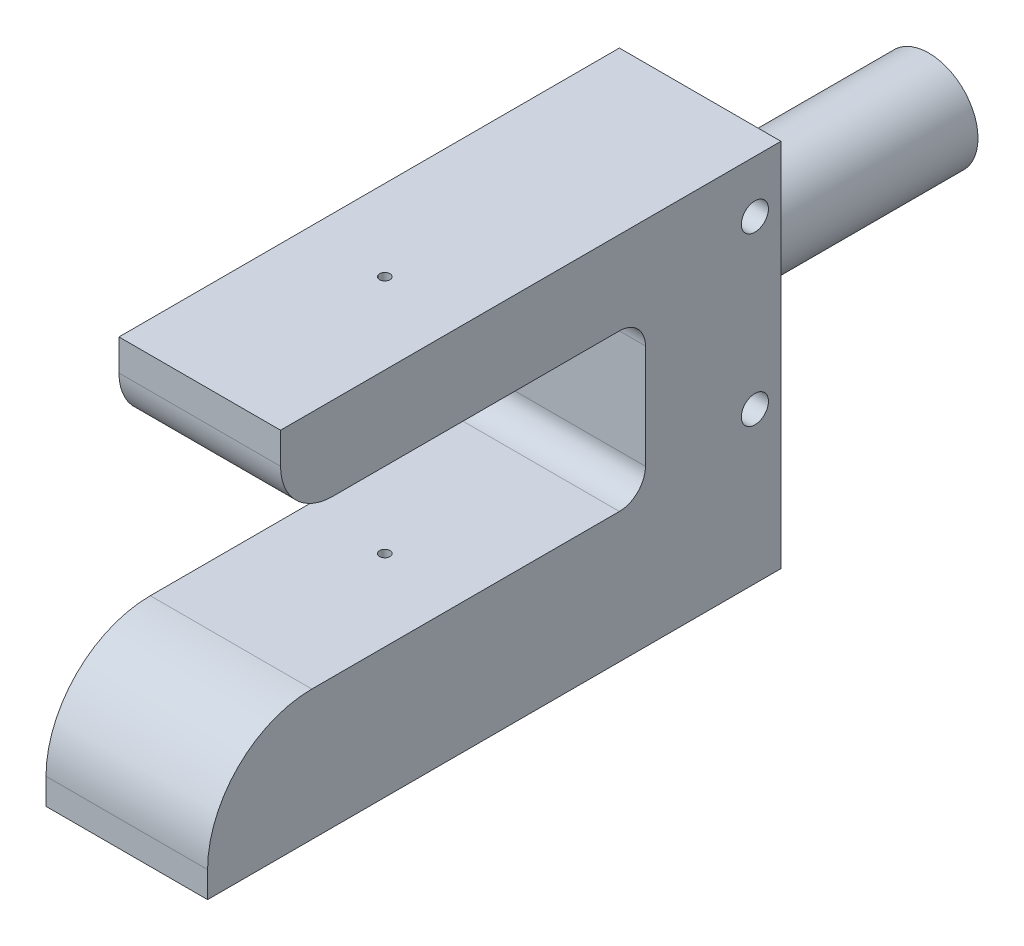
SolidWorks part; units mm, degrees
ref_plane "前视基准面" through (0, 0, 0) normal (0, 0, 1) x (1, 0, 0)
ref_plane "上视基准面" through (0, 0, 0) normal (0, 1, 0) x (1, 0, 0)
ref_plane "右视基准面" through (0, 0, 0) normal (1, 0, 0) x (0, 0, -1)
sketch "草图1" plane through (0, 0, 0) normal (1, 0, 0) x (0, 0, -1)
  line L0 (-55.3793, 24.9576) -> (14.6207, 24.9576)
  line L1 (-55.3793, 40.9576) -> (40.6207, 40.9576)
  line L2 (-55.3793, 40.9576) -> (-55.3793, 24.9576)
  line L3 (-69.3793, -30.0424) -> (40.6207, -30.0424)
  line L4 (40.6207, 40.9576) -> (40.6207, -30.0424)
  line L5 (-55.3793, 40.9576) -> (40.6207, -30.0424) construction
  line L6 (-38.0184, -38.3337) -> (40.6207, 40.9576) construction
  line L7 (14.6207, 24.9576) -> (14.6207, -5.0424)
  line L8 (14.6207, -5.0424) -> (-69.3793, -5.0424)
  line L9 (-69.3793, -5.0424) -> (-69.3793, -30.0424)
  point P0 (0, 0)
  dimension "D1" = 110
  dimension "D2" = 96
  dimension "D3" = 71
  dimension "D4" = 30
  dimension "D5" = 16
  dimension "D6" = 70
extrude "凸台-拉伸1" add sketch "草图1" along normal blind 31
sketch "草图2" plane through (0, 40.9576, 0) normal (0, 1, 0) x (1, 0, 0)
  line L0 (15.5, -69.3793) -> (15.5, 5.5421) construction
  line L1 (31, -69.3793) -> (0, -69.3793) construction
  line L2 (31, -55.3793) -> (0, -55.3793) construction
  circle A0 centre (15.5, -19.8793) radius 1
  dimension "D2" = 2
  dimension "D1" = 35.5
extrude "切除-拉伸1" cut sketch "草图2" against normal through all
fillet "圆角1" radius 10 1 edges at (15.5, 24.9576, 55.3793)
fillet "圆角2" radius 20 1 edges at (15.5, -5.0424, 69.3793)
fillet "圆角3" radius 5 2 edges at (15.5, -5.0424, -14.6207) (15.5, 24.9576, -14.6207)
hole_wizard "Ø5.2 (5.2) 直径孔1" positions "草图3" profile "草图4" hole size "Ø5.2" standard "GB"
sketch "草图3" plane through (31, 0, 0) normal (1, 0, 0) x (0, 0, -1)
  line L0 (40.6207, -30.0424) -> (40.6207, 40.9576) construction
  line L1 (40.6207, 40.9576) -> (-55.3793, 40.9576) construction
  point P0 (35.6207, 30.9576)
  point P2 (35.6207, -1.0424)
  dimension "D1" = 5
  dimension "D2" = 32
  dimension "D3" = 10
sketch "草图4" plane through (31, 30.9576, -35.6207) normal (0, 1, 0) x (0, 0, -1)
  line L0 (0, 0) -> (0, 64.5622)
  line L1 (0, 64.5622) -> (2.6, 63)
  line L2 (2.6, 63) -> (2.6, 0)
  line L5 (2.6, 0) -> (0, 0)
  line L10 (0, 64.5622) -> (-2.6, 63) construction
  line L11 (0, -6.35) -> (0, 107.95) construction
  dimension "孔直径" = 5.2
  dimension "孔深度" = 63
  dimension "导头角度" = 118
hole_wizard "M6 螺纹孔1" positions "草图5" profile "草图6" tap size "M6" standard "GB"
sketch "草图5" plane through (0, 0, -40.6207) normal (0, 0, -1) x (-1, 0, 0)
  line L2 (-15.5, -30.0424) -> (-15.5, 6.6482) construction
  line L3 (-31, -30.0424) -> (0, -30.0424) construction
  point P0 (-15.5, -13.0424)
  dimension "D1" = 17
sketch "草图6" plane through (15.5, -13.0424, -40.6207) normal (1, 0, 0) x (0, 1, 0)
  line L0 (0, 0) -> (0, 9.5022)
  line L1 (0, 9.5022) -> (2.5, 8)
  line L2 (2.5, 8) -> (2.5, 0)
  line L5 (2.5, 0) -> (0, 0)
  line L10 (0, 9.5022) -> (-2.5, 8) construction
  line L11 (0, -6.35) -> (0, 107.95) construction
  dimension "螺纹孔钻头直径" = 5
  dimension "螺纹孔钻头深度" = 8
  dimension "导头角度" = 118
cosmetic thread "孔螺蚊线1" parameters "D1"=8, "D2"=6
sketch "草图7" plane through (0, 0, -40.6207) normal (0, 0, -1) x (-1, 0, 0)
  circle A0 centre (-15.3708, 16.3775) radius 9.4338
extrude "凸台-拉伸2" add sketch "草图7" along normal blind 44
